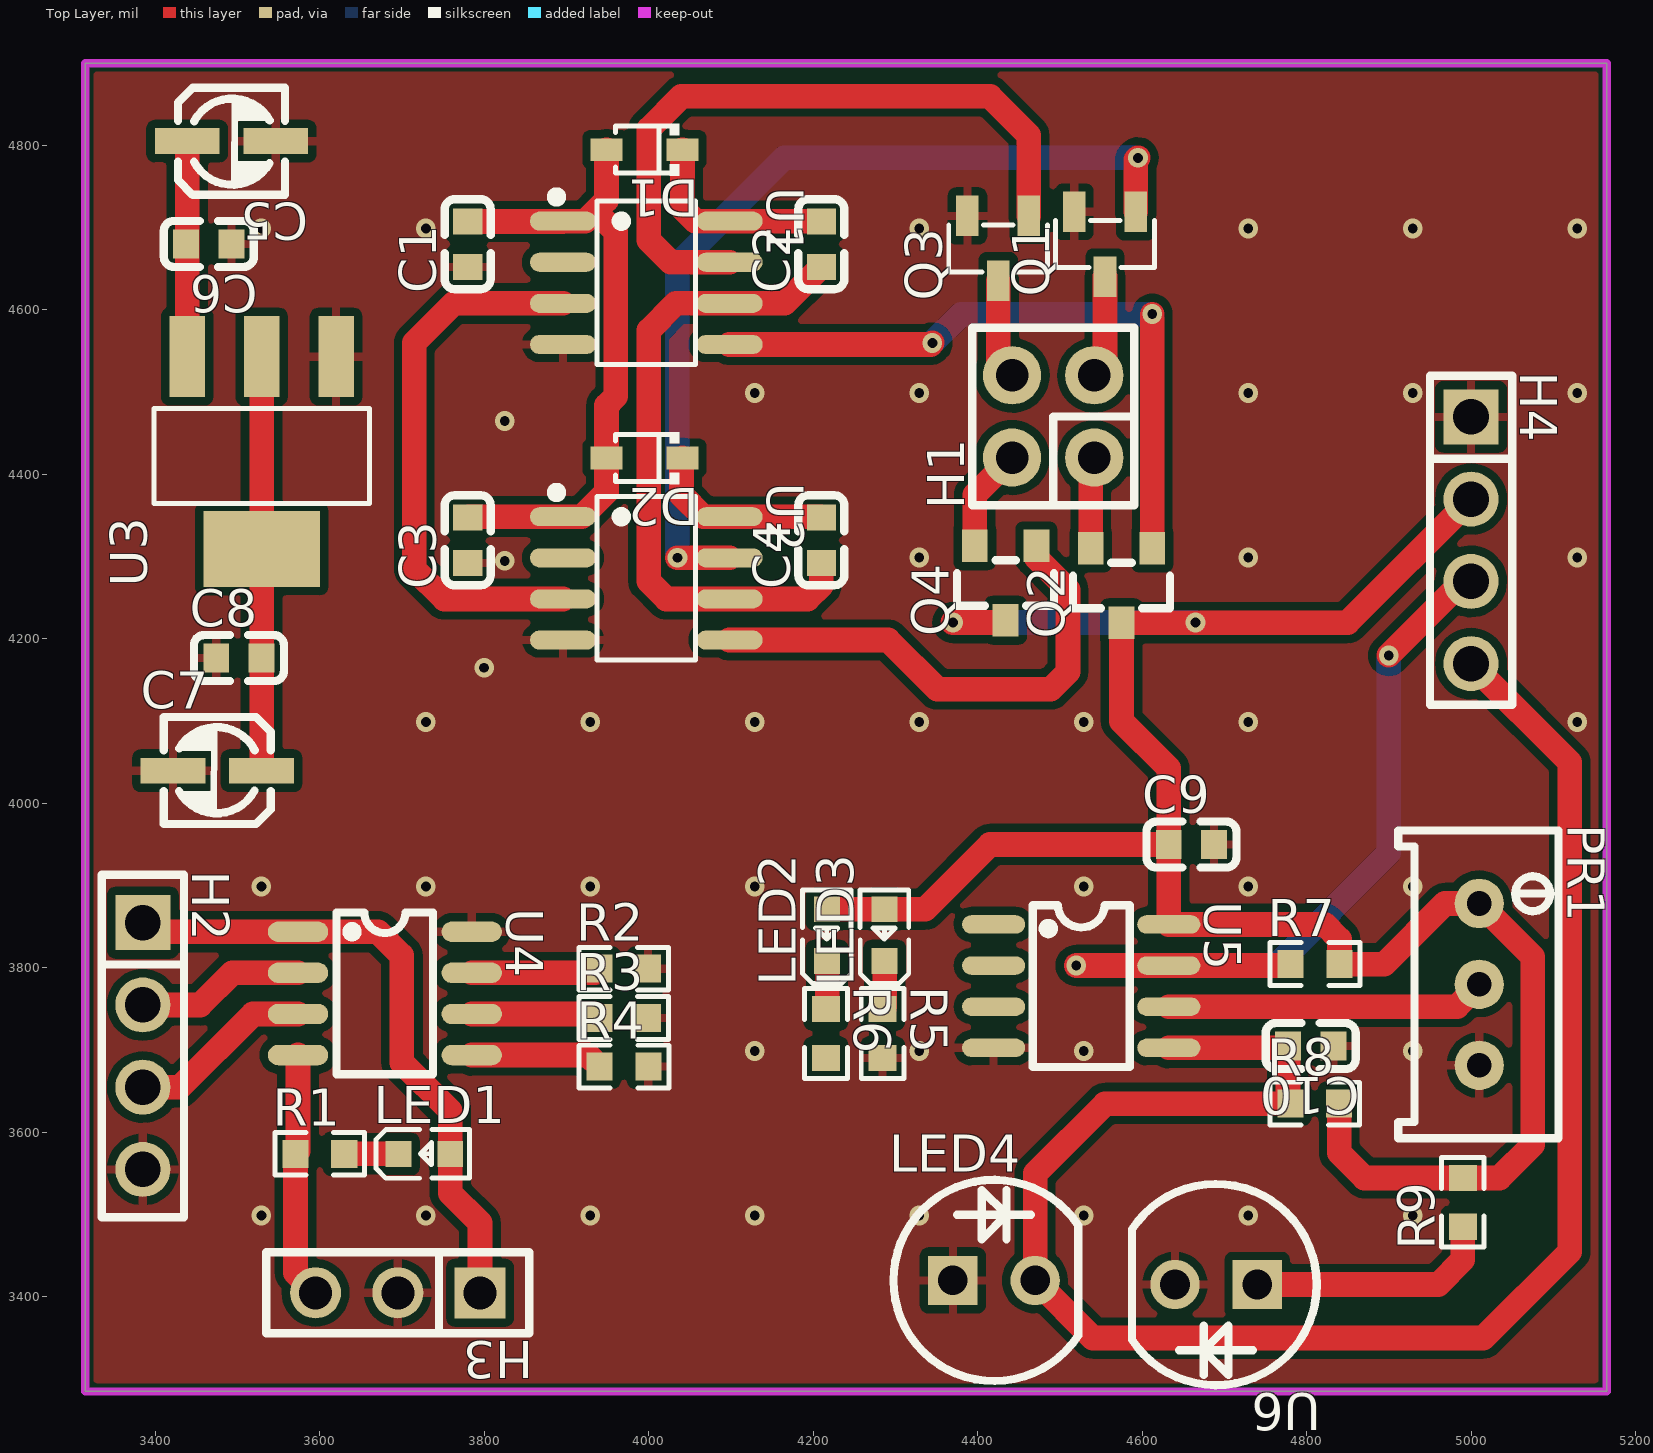
[diagram p0: Top Layer view]
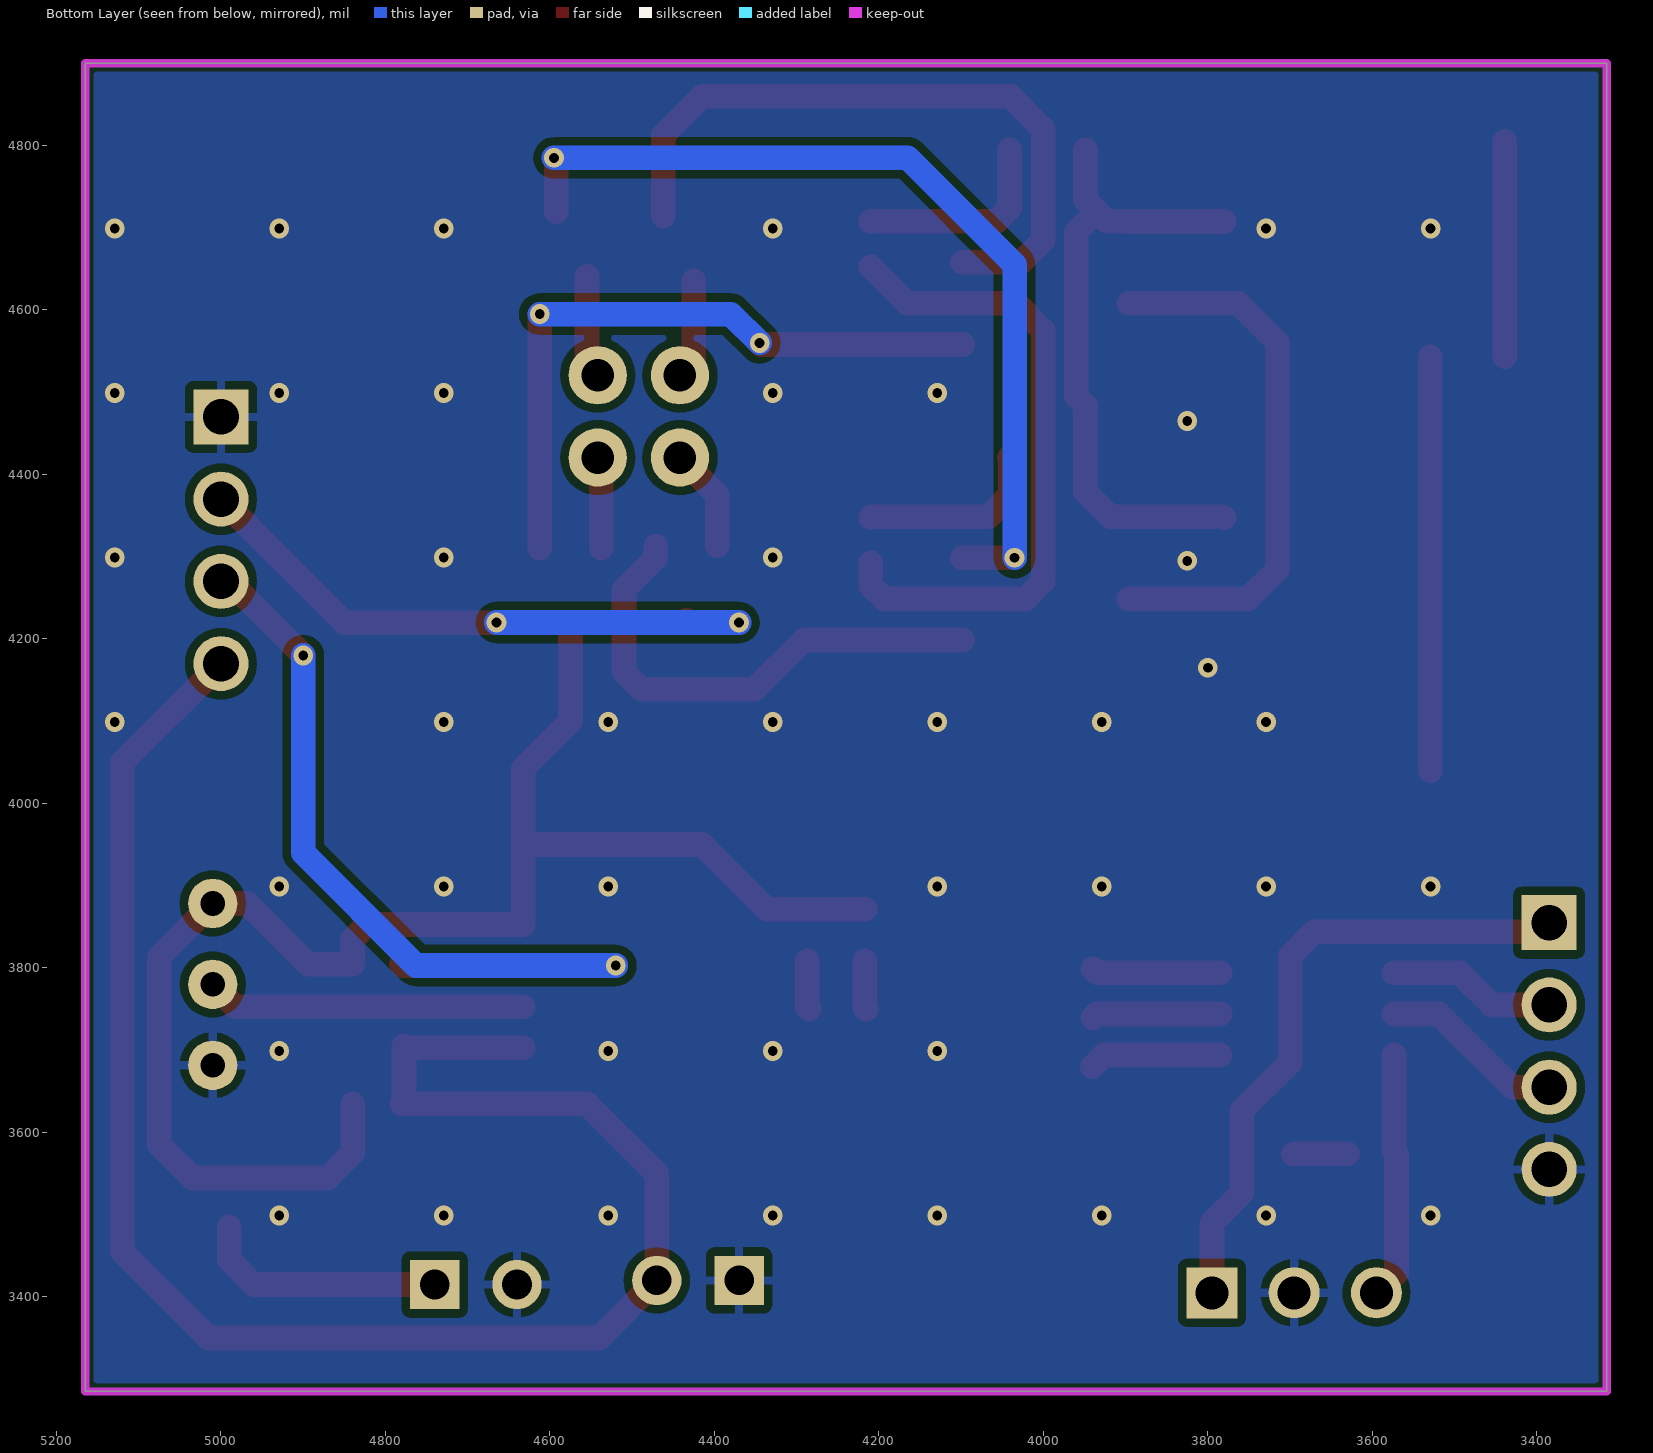
[diagram p1: Bottom Layer view, seen from below]
# Altium PCB MISC64784.pcbdoc
Units mil, origin at the board's own origin, x right, y up, seen from the top; angles counter-clockwise.
Board outline 1850 x 1615 mil, 2 copper layers (Top Layer, Bottom Layer), stack 62.206 mil thick; 40 components, 34 nets, 118 pads, 51 vias.

## Layer stack, top to bottom
Top Solder Mask Layer: solder mask 0.394, Dk 3.3
Top Layer: signal copper 1.379
Dielectric1: surface 59.449, FR4, Dk 4.5
Bottom Layer: signal copper 1.378
Bottom Solder Mask Layer: solder mask 0.394, Dk 3.3

## Board outline
3315,4900 3315,3285 5165,3285 5165,4900

## Design rules (kind name [scope] priority, off if disabled: settings)
BoardOutlineClearance copperThickness2oz_1 [All] p2 off: genericclearance=7.99 ignorepadtopadclearanceinfootprint=FALSE except(0: Arc-SplitContinuation Track-SplitContinuation SMDPad-SplitContinuation THPad-SplitContinuation Via-SplitContinuation Fill-SplitContinuation Region-SplitContinuation Poly-SplitContinuation Text-SplitContinuation Hole-SplitContinuation; 5.98: Arc-CutoutEdge SMDPad-CutoutEdge THPad-CutoutEdge Via-CutoutEdge Fill-CutoutEdge Region-CutoutEdge Text-CutoutEdge; 6.93: Hole-OutlineEdge Hole-CutoutEdge; 10: Poly-OutlineEdge Poly-CutoutEdge; 11.81: Arc-OutlineEdge Track-OutlineEdge SMDPad-OutlineEdge THPad-OutlineEdge Via-OutlineEdge Fill-OutlineEdge Region-OutlineEdge Text-OutlineEdge Track-CutoutEdge)
BoardOutlineClearance copperThickness1oz_1 [All] p4: genericclearance=4.02 ignorepadtopadclearanceinfootprint=FALSE except(0: Arc-SplitContinuation Track-SplitContinuation SMDPad-SplitContinuation THPad-SplitContinuation Via-SplitContinuation Fill-SplitContinuation Region-SplitContinuation Poly-SplitContinuation Text-SplitContinuation Hole-SplitContinuation; 6: SMDPad-CutoutEdge THPad-CutoutEdge Via-CutoutEdge Fill-CutoutEdge Region-CutoutEdge Text-CutoutEdge; 6.93: Hole-OutlineEdge Hole-CutoutEdge; 10: Poly-OutlineEdge Poly-CutoutEdge; 11.8: Arc-OutlineEdge Track-OutlineEdge SMDPad-OutlineEdge THPad-OutlineEdge Via-OutlineEdge Fill-OutlineEdge Region-OutlineEdge Text-OutlineEdge; 11.81: Arc-CutoutEdge Track-CutoutEdge)
Clearance copperThickness2oz [All] p1 off: gap=7.99 ignorepadtopadclearanceinfootprint=FALSE except(5.98: SMDPad-Track SMDPad-SMDPad THPad-Track SMDPad-THPad THPad-THPad Track-Via SMDPad-Via THPad-Via Via-Via Fill-Track Region-Track Fill-SMDPad Region-SMDPad Fill-THPad Region-THPad Fill-Via Region-Via Fill-Fill Fill-Region Region-Region Arc-Track Arc-SMDPad Arc-THPad Arc-Via Fill-Arc Region-Arc Arc-Arc Text-Track SMDPad-Text Text-THPad Text-Via Fill-Text Region-Text Arc-Text Text-Text; 6.93: Hole-Track Hole-SMDPad Hole-THPad Hole-Via Fill-Hole Region-Hole Hole-Arc Hole-Text; 10: Poly-Track Poly-SMDPad Poly-THPad Poly-Via Poly-Fill Poly-Region Poly-Poly Poly-Arc Poly-Text Poly-Hole)
Clearance copperThickness1oz [All] p3: gap=4.02 ignorepadtopadclearanceinfootprint=FALSE except(5.98: SMDPad-Track SMDPad-SMDPad THPad-Track SMDPad-THPad THPad-THPad Track-Via SMDPad-Via THPad-Via Via-Via Fill-Track Region-Track Fill-SMDPad Region-SMDPad Fill-THPad Region-THPad Fill-Via Region-Via Fill-Fill Fill-Region Region-Region; 6: Arc-Track Arc-SMDPad Arc-THPad Arc-Via Fill-Arc Region-Arc Arc-Arc Text-Track SMDPad-Text Text-THPad Text-Via Fill-Text Region-Text Arc-Text Text-Text; 6.93: Hole-Track Hole-SMDPad Hole-THPad Hole-Via Fill-Hole Region-Hole Hole-Arc Hole-Text; 10: Poly-Track Poly-SMDPad Poly-THPad Poly-Via Poly-Fill Poly-Region Poly-Poly Poly-Arc Poly-Text Poly-Hole)
DiffPairsRouting differentialPair [All] p1: maxlimit=6 minlimit=6 mostfreqgap=6 toplayer_minwidth=5 toplayer_prefwidth=10 toplayer_maxwidth=100 toplayer_mingap=6 toplayer_prefgap=6 toplayer_maxgap=6 bottomlayer_minwidth=5 bottomlayer_prefwidth=10 bottomlayer_maxwidth=100 bottomlayer_mingap=6 bottomlayer_prefgap=6 bottomlayer_maxgap=6 maxuncoupledlength=10
HoleToHoleClearance otherClearance [All] p1: gap=11.81 allowstackedmicrovias=TRUE
Length netLength [All] p1: minlimit=0 maxlimit=0
MatchedLengths netLengthTolerance [All] p1: tolerance=1000
PasteMaskExpansion pasteMaskExpansion [All] p1: expansion=0
PlaneConnect innerPlane [All] p1: planeconnectstyle=Relief reliefexpansion=20 reliefentries=4 reliefconductorwidth=10 reliefairgap=10
PolygonConnect copperRegion [(InNet('GND'))] p1: connectstyle=Relief reliefconductorwidth=10 reliefentries=4 polygonreliefangle="90 Angle" airgapwidth=10 via.connectstyle=Relief via.reliefconductorwidth=10 via.reliefentries=4 via.polygonreliefangle="90 Angle" via.airgapwidth=10
RoutingVias viaSize [All] p1: holewidth=12.01 width=24.02 viastyle="Through Hole" minholewidth=11.81 minwidth=19.68 maxholewidth=248.03 maxwidth=393.7
SolderMaskExpansion solderMaskExpansion [IsVia] p1: expansion=-1000 istentingtop=TRUE
SolderMaskExpansion solderMaskExpansion [All] p2: expansion=2 istentingtop=FALSE
Width copperThickness2oz_2 [All] p1 off: maxlimit=100 minlimit=8 preferedwidth=10
Width copperThickness1oz_2 [All] p2: maxlimit=100 minlimit=5 preferedwidth=10

## Components (designator, comment, footprint, x,y, rotation, side; value= is the part's Value field where it differs from the comment)
C1 "100nF" C0603 3780,4680 r90 top
C2 "100nF" C0603 4210,4680 r90 top
C3 "100nF" C0603 3780,4320 r90 top
C4 "100nF" C0603 4210,4320 r90 top
C5 "10uF" C_Ele_SMD_3x5.4mm 3492.99,4804.75 r180 top
C6 "100nF" C0603 3465.25,4680.34 r180 top
C7 "10uF" C_Ele_SMD_3x5.4mm 3475.25,4040.34 r0 top
C8 "100nF" C0603 3501.88,4176.78 r0 top
C9 "100nF" C0603 4660,3950 r0 top
C10 "100nF" C0603 4805,3705 r180 top
D1 "1N5819WS" SOD-323_L1.8-W1.3-LS2.5-RD 3995,4795 r180 top
D2 "1N5819WS" SOD-323_L1.8-W1.3-LS2.5-RD 3995,4420 r180 top
H1 "" HDR-TH_4P-P2.54-V-F-R2-C2-S2.54 4491.94,4470.56 r90 top
H2 "" HDR-TH_4P-P2.54-V-F 3385,3705 r270 top
H3 "" HDR-TH_3P-P2.54-V-F 3695,3405 r180 top
H4 "" HDR-TH_4P-P2.54-V-M 5000,4320 r270 top
LED1 "" LED_0603 3729.29,3573.98 r0 top
LED2 "" LED_0603 4216.64,3841.84 r90 top
LED3 "" LED_0603 4286.64,3841.84 r90 top
LED4 "PT334-6B" LED-TH_BD5.9-P2.54-FD 4420,3420 r0 top
PR1 "10kΩ" R_3296 5015,3780 r270 top
Q1 "" SOT-23-3_L2.9-W1.3-P1.90-LS2.4-BR 4555,4680 r90 top
Q2 "" AO3401A_SOT-23-3 4575,4265 r90 top
Q3 "" SOT-23-3_L2.9-W1.3-P1.90-LS2.4-BR 4425,4675 r90 top
Q4 "" AO3401A_SOT-23-3 4434.01,4268.06 r90 top
R1 "1K" R0603 3600.21,3573.98 r0 top
R2 "NC" R0603 3969.74,3799.02 r0 top
R3 "NC" R0603 3969.74,3739.02 r0 top
R4 "NC" R0603 3970,3680 r0 top
R5 "1K" R0603 4284.52,3720.24 r270 top
R6 "1K" R0603 4215.63,3720.24 r270 top
R7 "10K" R0603 4810.34,3804.66 r0 top
R8 "10K" R0603 4810,3635 r0 top
R9 "100" R0603 4990,3515 r90 top
U1 "IR2104STRPBF" SOIC-8_L4.9-W3.9-P1.27-LS6.0-BL 3997.12,4633.05 r270 top
U2 "IR2104STRPBF" SOIC-8_L4.9-W3.9-P1.27-LS6.0-BL 3997.12,4273.67 r270 top
U3 "AMS1117-3.3" SOT-223-3_L6.5-W3.4-P2.30-LS7.0-BR 3529.44,4426.34 r90 top
U4 "1152" SOP-8_L4.9-W3.9-P1.27-LS6.0-BL 3679.34,3769.02 r270 top
U5 "LM393DT" SOIC-8_L5.0-W4.0-P1.27-LS6.0-BL 4526,3777.88 r270 top
U6 "DY-IR333C-A" LED-TH_BD5.9-P2.54-FD 4690,3415 r180 top

## Footprints (in the part's own frame and the unit in brackets; to place one, negate y for a bottom-side part, rotate by r counter-clockwise, add the part's x,y. Pads: shape width x height; smd on the part's side, far side on the other; paste and mask are expansions set on the pad)
AO3401A_SOT-23-3 [mm]
  rect 1x0.8 smd paste+0 mask+0.051: 1(1.15,-0.95) 2(1.15,0.95) 3(-1.15,0)
  silkscreen extent -0.7,-1.5 0.7,1.5
C0603 [mm]
  rect 0.8x0.9 smd: 1(-0.7,0) 2(0.7,0)
  silkscreen extent -1.39,-0.71 1.39,0.71
C_Ele_SMD_3x5.4mm [mil]
  rect 78.7x31.5 smd paste+0 mask+2: 1(54.1,-0.55) 2(-53.7,-0.55)
  silkscreen extent -65,-65 65,65
HDR-TH_3P-P2.54-V-F [mil]
  rect 62x62 hole 40.16: 1(-100,0)
  round 62 hole 40.16: 2(0,0) 3(100,0)
  silkscreen extent -160,-49 160,49
HDR-TH_4P-P2.54-V-F [mm]
  rect 1.7x1.7 hole 1.1: 1(-3.81,0)
  round 1.7 hole 1.1: 2(-1.27,0) 3(1.27,0) 4(3.81,0)
  silkscreen extent -5.29,-1.27 5.29,1.27
HDR-TH_4P-P2.54-V-F-R2-C2-S2.54 [mm]
  round 1.8 hole 1: 1(-1.27,-1.27) 2(-1.27,1.27) 3(1.27,-1.27) 4(1.27,1.27)
  silkscreen extent -2.74,-2.5 2.74,2.5
HDR-TH_4P-P2.54-V-M [mm]
  rect 1.7x1.7 hole 1.1: 1(-3.81,0)
  round 1.7 hole 1.1: 2(-1.27,0) 3(1.27,0) 4(3.81,0)
  silkscreen extent -5.08,-1.27 5.08,1.27
LED-TH_BD5.9-P2.54-FD [mil]
  rect 60x60 hole 36: 1(-50,0)
  round 60 hole 36: 2(50,0)
  silkscreen extent -122,-122 102,122
LED_0603 [mil]
  rect 31.5x31.5 smd paste+0 mask+2: 1(-33.5,-0.4) 2(29.5,-0.2)
  silkscreen extent -61,-30 53,30
R0603 [mil]
  rect 31.75x34.02 smd paste-3937.01 mask+2: 1(-29.66,0) 2(29.66,0)
  silkscreen extent -55,-26 55,26
R_3296 [mil]
  round 60 hole 30 paste+0 mask+2: 1(-98.4,-5) 2(0,-5) 3(98.4,-5)
  silkscreen extent -187,-103 187,92
SOD-323_L1.8-W1.3-LS2.5-RD [mm]
  rect 1x0.7 smd: 1(-1.172,0) 2(1.172,0)
  silkscreen extent -1.08,-0.8 0.9,0.8
SOIC-8_L4.9-W3.9-P1.27-LS6.0-BL [mm]
  oval 0.588x2.045 smd: 1(-1.905,-2.57) 2(-0.635,-2.57) 3(0.635,-2.57) 4(1.905,-2.57) 5(1.905,2.57) 6(0.635,2.57) 7(-0.635,2.57) 8(-1.905,2.57)
  silkscreen extent -2.8,-2.92 2.53,1.52
SOIC-8_L5.0-W4.0-P1.27-LS6.0-BL [mil]
  oval 22.38x76.78 smd: 1(-75,-106.5) 2(-25,-106.5) 3(25,-106.5) 4(75,-106.5) 5(75,106.5) 6(25,106.5) 7(-25,106.5) 8(-75,106.5)
  silkscreen extent -98,-59 98,59
SOP-8_L4.9-W3.9-P1.27-LS6.0-BL [mm]
  oval 0.63x1.865 smd: 1(-1.905,-2.682) 2(-0.635,-2.682) 3(0.635,-2.682) 4(1.905,-2.682) 5(1.905,2.682) 6(0.635,2.682) 7(-0.635,2.682) 8(-1.905,2.682)
  silkscreen extent -2.5,-1.5 2.5,1.48
SOT-23-3_L2.9-W1.3-P1.90-LS2.4-BR [mm]
  rect 1.25x0.7 smd: 1(1,-0.95) 2(1,0.95) 3(-1,0)
  silkscreen extent -0.73,-1.53 0.73,1.53
SOT-223-3_L6.5-W3.4-P2.30-LS7.0-BR [mm]
  rect 2.5x1.1 smd: 1(2.97,-2.3) 2(2.97,0) 3(2.97,2.3)
  rect 2.34x3.6 smd: 4(-2.97,0)
  silkscreen extent -1.57,-3.33 1.37,3.33

## Via types
v1: diameter 24.02, hole 12, Top Layer to Bottom Layer, 51 vias

## Nets (pads, with @x,y where several pads share a name; then routed paths per layer and width w, separated by ;. In a path a pad name is that pad's centre, name@x,y a point inside that pad or via, vN(x,y) a via of type N, cw(c..) or ccw(c..) an arc to the next point about the centre after c; other vN are vias at no path point)
3V3: C7.1 C8.2 U3.2 U3.4 | length 503.5
  Top Layer w30: C7.1 3529.44,4039.89 C8.2 U3.4 U3.2
5V: C5.1 C6.2 U3.3 | length 262
  Top Layer w30: U3.3 C5.1
$1N8: C2.2 D1.1 U1.8 | length 246.7
  Top Layer w30: D1.1 4041.16,4723.84 4056.95,4708.05 U1.8 4209.51,4708.05 C2.2
$1N9: C4.2 D2.1 U2.8 | length 226.8
  Top Layer w30: D2.1 4040,4418.84 4040,4375 4066.33,4348.67 U2.8 4208.89,4348.67 C4.2
$1N21: H1.1 Q2.2 | length 112.1
  Top Layer w30: Q2.2 4537.6,4416.22 H1.1
$1N22: H1.3 Q1.3 | length 125.5
  Top Layer w30: H1.3 4555,4533.62 Q1.3
$1N31: H1.4 Q3.3 | length 122.1
  Top Layer w30: Q3.3 4425,4537.5 H1.4
$1N32: H1.2 Q4.2 | length 126
  Top Layer w30: Q4.2 4396.61,4375.23 H1.2
$1N45: H3.3 R1.1 U4.4 | length 300.5
  Top Layer w30: U4.4 3573.74,3577.17 R1.1 3570.55,3429.45 H3.3
$1N46: LED1.1 R1.2 | length 66.1
  Top Layer w30: R1.2 3695.39,3573.98 LED1.1
$1N49: R2.1 U4.7 | length 157.2
  Top Layer w30: U4.7 3935.08,3794.02 R2.1
$1N50: R3.1 U4.6 | length 157.2
  Top Layer w30: U4.6 3935.08,3744.02 R3.1
$1N52: R4.1 U4.5 | length 161.2
  Top Layer w30: U4.5 3926.32,3694.02 R4.1
$1N54: LED3.1 R5.1 | length 59.5
  Top Layer w30: R5.1 4287.04,3752.42 LED3.1
$1N55: LED2.1 R6.1 | length 59
  Top Layer w30: R6.1 4217.04,3751.32 LED2.1
$1N63: H4.3 R7.1 U5.7 | length 1075.5
  Top Layer w30: v1(4520,3802.88) U5.7 4778.9,3802.88 R7.1 ; v1(4900,4180) 4990,4270 H4.3
  Bottom Layer w30: v1(4520,3802.88) 4762.88,3802.88 4900,3940 v1(4900,4180)
$1N68: PR1.2 U5.6 | length 388.7
  Top Layer w30: U5.6 4982.88,3752.88 PR1.2
$1N76: R9.1 U6.1 | length 302.8
  Top Layer w30: U6.1 4960,3415 4990,3445 R9.1
+3.3V: H2.1 H3.1 LED1.2 U4.1 | length 780.9
  Top Layer w30: H2.1 3395.98,3844.02 U4.1 3670.98,3844.02 3700,3815 3700,3685 3758.79,3626.21 LED1.2 3758.79,3526.21 3795,3490 H3.1
+15V: C1.2 C3.2 D1.2 D2.2 U1.1 U2.1 | length 778.8
  Top Layer w30: C3.2 3781.11,4348.67 U2.1 3918.67,4348.67 3948.84,4378.84 D2.2 3948.84,4483.84 3960,4495 3960,4695 3935,4720 ; C1.2 3895.45,4707.56 U1.1 3923.05,4708.05 3935,4720 ; D1.2 3948.84,4733.84 3935,4720
AO: C10.2 H4.4 LED4.2 R8.1 U5.5 | length 2179.8
  Top Layer w30: U5.5 4775.32,3702.88 C10.2 4777.44,3637.9 R8.1 4555,3635 4470,3550 LED4.2 4540,3350 5015,3350 5120,3455 5120,4050 H4.4
D0: R6.2
ECHO: H2.3 U4.3 | length 225.6
  Top Layer w30: H2.3 3430,3655 3519.02,3744.02 U4.3
GND: C1.1 C3.1 C5.2 C6.1 C7.2 C8.1 C9.2 C10.1 H2.4 H3.2 H4.1 LED4.1 PR1.3 Q1.2 Q3.2 R2.2 R3.2 R4.2 R5.2 U1.4 U2.4 U3.1 U4.8 U5.4 U6.2
  other v1: 3529.1,3499.1 3729.1,3499.1 3929.1,3499.1 4129.1,3499.1 4329.1,3499.1 4529.1,3499.1 4729.1,3499.1 4929.1,3499.1 4129.1,3699.1 4329.1,3699.1 4529.1,3699.1 4929.1,3699.1 3529.1,3899.1 3729.1,3899.1 3929.1,3899.1 4129.1,3899.1 4529.1,3899.1 4729.1,3899.1 4929.1,3899.1 3729.1,4099.1 3929.1,4099.1 4129.1,4099.1 4329.1,4099.1 4529.1,4099.1 4729.1,4099.1 5129.1,4099.1 3800,4165 3825,4295 4329.1,4299.1 4729.1,4299.1 5129.1,4299.1 3825,4465 4129.1,4499.1 4329.1,4499.1 4729.1,4499.1 4929.1,4499.1 5129.1,4499.1 3529.1,4699.1 3729.1,4699.1 4329.1,4699.1 4729.1,4699.1 4929.1,4699.1 5129.1,4699.1
MOS1-H: Q2.1 U1.5 | length 814.1
  Top Layer w30: U1.5 4343.05,4558.05 v1(4345,4560) ; Q2.1 v1(4612.4,4595)
  Bottom Layer w30: v1(4345,4560) 4380,4595 v1(4612.4,4595)
MOS1-L: Q3.1 U1.7 | length 841.3
  Top Layer w30: U1.7 4026.95,4658.05 4000,4685 4000,4820 4040,4860 4415,4860 4462.4,4812.6 Q3.1
MOS2-H: Q4.1 U2.5 | length 614.6
  Top Layer w30: U2.5 4291.33,4198.67 4351.21,4138.79 4488.79,4138.79 4510,4160 4510,4260 4471.41,4298.59 Q4.1
MOS2-L: Q1.1 U2.7 | length 1100.2
  Top Layer w30: v1(4035,4298.67) U2.7 ; Q1.1 4592.4,4782.4 v1(4595,4785)
  Bottom Layer w30: v1(4035,4298.67) 4035,4655 4165,4785 v1(4595,4785)
PA1: U1.3 U2.3 | length 671.8
  Top Layer w30: U2.3 3751.33,4248.67 3715,4285 3715,4560 3763.05,4608.05 U1.3
PA2: U2.2
PC13: U1.2
TRIG: H2.2 U4.2 | length 204.9
  Top Layer w30: H2.2 3455,3755 3494.02,3794.02 U4.2
VCC: C9.1 H4.2 LED2.2 LED3.2 PR1.1 Q2.3 Q4.3 R7.2 R8.2 R9.2 U5.8 | length 2776.7
  Top Layer w30: LED2.2 LED3.2 4336.34,3871.34 4415,3950 C9.1 4632.44,4042.56 4575,4100 Q2.3 4849.72,4219.72 H4.2 ; v1(4370,4220) 4431.22,4220 Q4.3 ; C9.1@4632.5,3949.94 U5.8 4822.12,3852.88 4840,3835 R7.2 4894.66,3804.66 4968.4,3878.4 PR1.1 5075,3813.4 5075,3585 5034.66,3544.66 R9.2 4870.34,3544.66 4839.66,3575.34 R8.2
  Bottom Layer w30: v1(4370,4220) v1(4665,4220)
VS: C2.1 C4.1 U1.6 U2.6 | length 800.1
  Top Layer w30: C4.1 4210,4265 4193.67,4248.67 U2.6 4021.33,4248.67 4000,4270 4000,4575 4033.05,4608.05 U1.6 4165.61,4608.05 C2.1
pads on no net: U5.1 U5.2 U5.3

## Polygon pours and split planes (outlines as drawn)
GND on Top Layer (solid, remove dead copper, pour order 0): 3000,5115 3000,3000 5375,3000 5375,5115
GND on Bottom Layer (solid, remove dead copper, pour order 2): 3205,5040 3205,3075 5455,3075 5455,5040

## Keep-outs
Board Outline Layer:
  the board outline again, w10